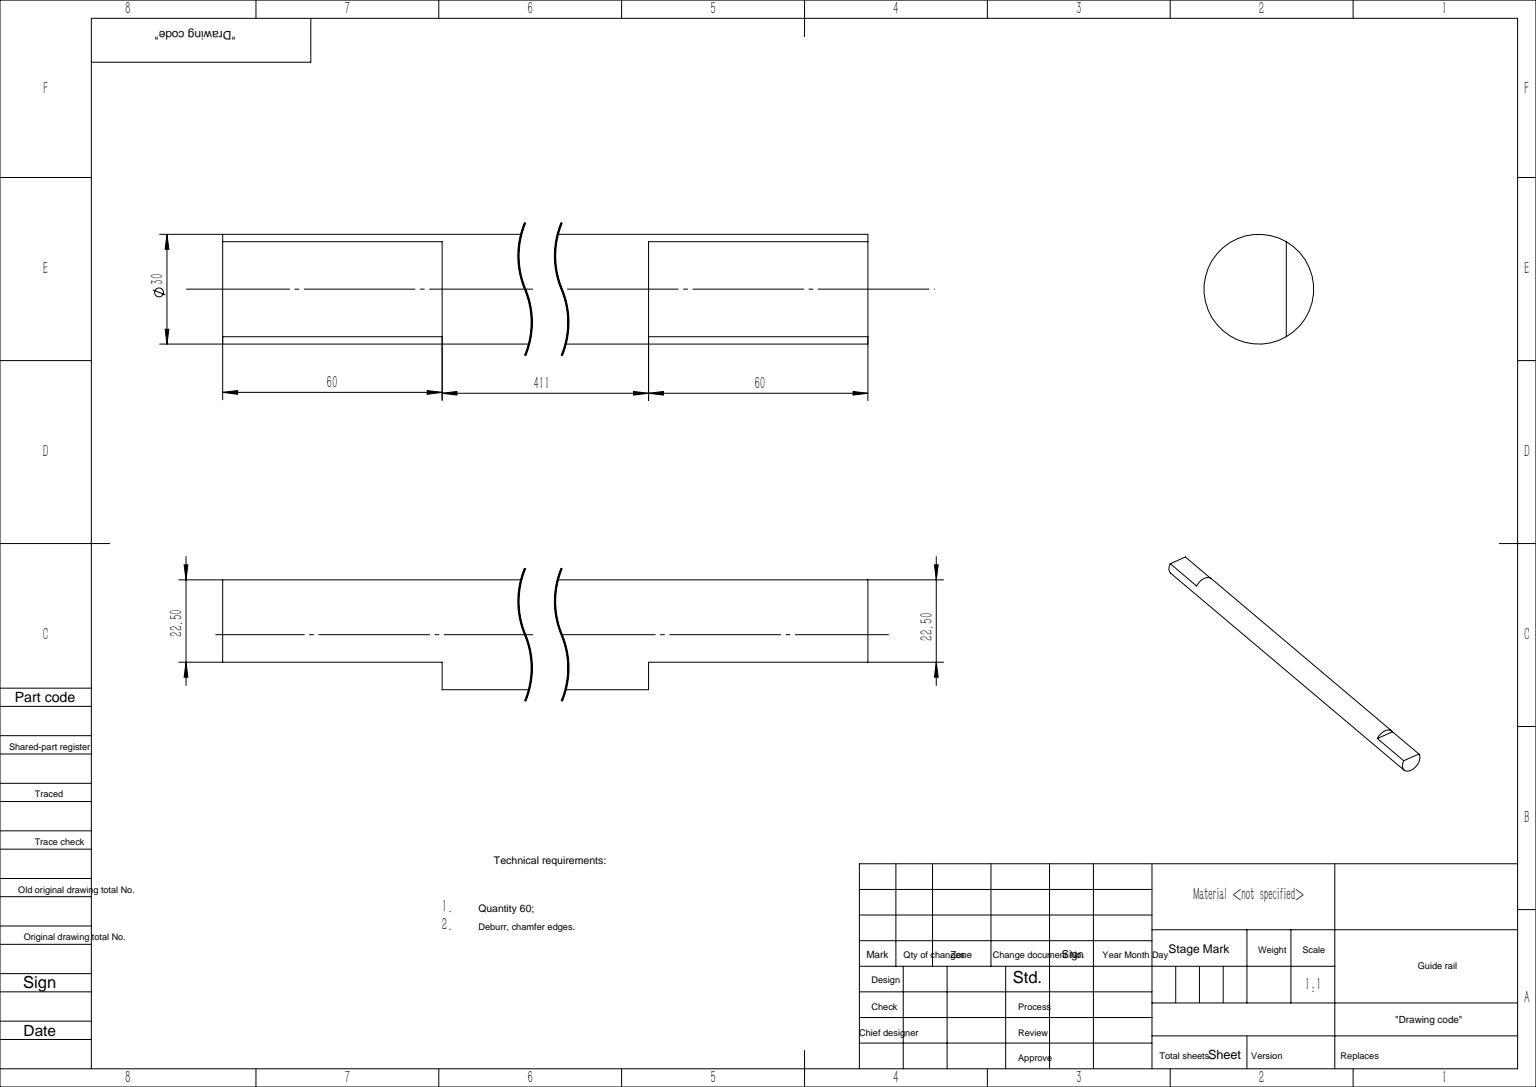
SolidWorks part; units mm, degrees
ref_plane "前视基准面" through (0, 0, 0) normal (0, 0, 1) x (1, 0, 0)
ref_plane "上视基准面" through (0, 0, 0) normal (0, 1, 0) x (1, 0, 0)
ref_plane "右视基准面" through (0, 0, 0) normal (1, 0, 0) x (0, 0, -1)
sketch "草图1" plane through (0, 0, 0) normal (0, 1, 0) x (1, 0, 0)
  circle A0 centre (0, 0) radius 15
  dimension "D1" = 30
extrude "凸台-拉伸1" add sketch "草图1" along normal blind 531
sketch "草图2" plane through (0, 531, 0) normal (0, 1, 0) x (1, 0, 0)
  line L0 (7.5, 12.9904) -> (7.5, -12.9904)
  arc A0 (7.5, -12.9904) -> (7.5, 12.9904) centre (0, 0) ccw
  circle A1 centre (0, 0) radius 15 construction
  dimension "D1" = 7.5
extrude "切除-拉伸1" cut sketch "草图2" against normal blind 60
ref_plane "基准面1" through (0, 265.5, 0) normal (0, 1, 0) x (1, 0, 0)
mirror "镜向1" about plane through (0, 265.5, 0) normal (0, 1, 0) of "切除-拉伸1"
